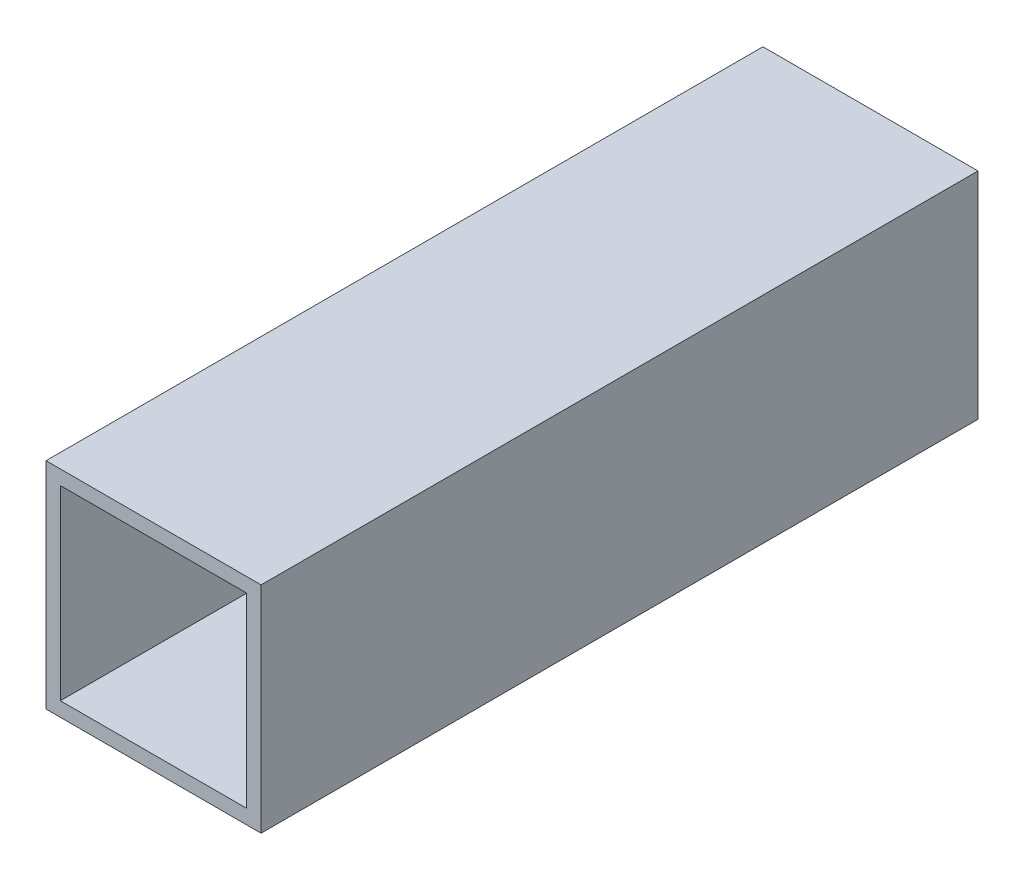
from build123d import *

# Parameters (mm, degrees)
SKETCH_1_W      = 30
SKETCH_1_H      = 30
SKETCH_1_W_2    = 26
SKETCH_1_H_2    = 26
EXTRUDE_1_DEPTH = 50


with BuildPart() as part:
    # 草图1 → 凸台-拉伸1 (new, symmetric)
    with BuildSketch(Plane.XY):
        Rectangle(SKETCH_1_W, SKETCH_1_H)
        Rectangle(SKETCH_1_W_2, SKETCH_1_H_2, mode=Mode.SUBTRACT)
    extrude(amount=EXTRUDE_1_DEPTH, both=True)


solid = part.part
